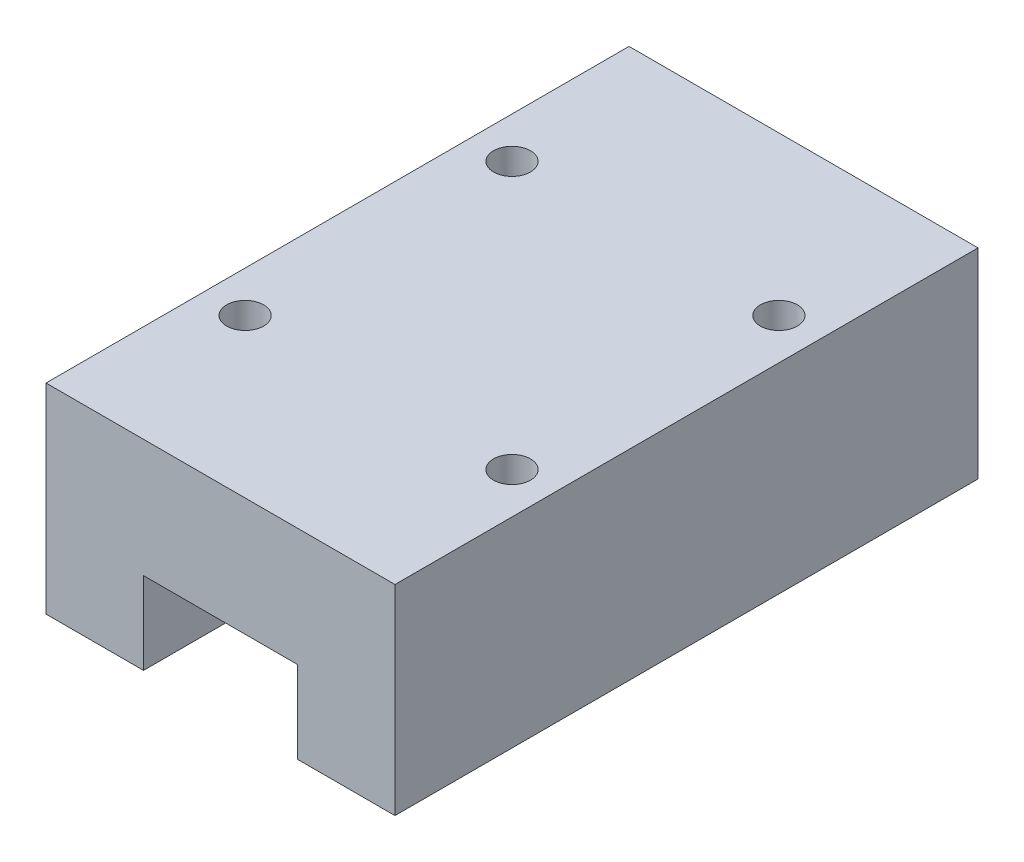
from build123d import *

# Parameters (mm, degrees)
SKETCH_1_W               = 34
SKETCH_1_H               = 19.5
EXTRUDE_1_DEPTH          = 28.4
CUT_EXTRUDE_1_DEPTH      = 35.505398128
CUT_EXTRUDE_1_DEPTH_BACK = 35.505398128
SKETCH_2_W               = 15
SKETCH_2_H               = 8
SKETCH_4_R               = 1.8
CUT_EXTRUDE_2_DEPTH      = 6


with BuildPart() as part:
    # 草图1 → 凸台-拉伸1 (new, symmetric)
    with BuildSketch(Plane.XY):
        Rectangle(SKETCH_1_W, SKETCH_1_H)
    extrude(amount=EXTRUDE_1_DEPTH, both=True)

    # 草图2 → 切除-拉伸1 (cut, two sides: drawn at the far end of the back side and taken through both)
    with BuildSketch(Plane.XY.offset(-CUT_EXTRUDE_1_DEPTH_BACK)):
        with Locations((0, -5.75)):
            Rectangle(SKETCH_2_W, SKETCH_2_H)
    extrude(amount=CUT_EXTRUDE_1_DEPTH + CUT_EXTRUDE_1_DEPTH_BACK, mode=Mode.SUBTRACT)

    # 草图4 → 切除-拉伸2 (cut)
    with BuildSketch(Plane(origin=(0, 9.75, 0), x_dir=(1, 0, 0), z_dir=(0, 1, 0))):
        with Locations(Location((-13, 13, 0), (0, 0, 270))):
            Circle(SKETCH_4_R)
        with Locations(Location((13, 13, 0), (0, 0, 90))):
            Circle(SKETCH_4_R)
        with Locations(Location((13, -13, 0), (0, 0, 270))):
            Circle(SKETCH_4_R)
        with Locations(Location((-13, -13, 0), (0, 0, 90))):
            Circle(SKETCH_4_R)
    extrude(amount=-CUT_EXTRUDE_2_DEPTH, mode=Mode.SUBTRACT)


solid = part.part
